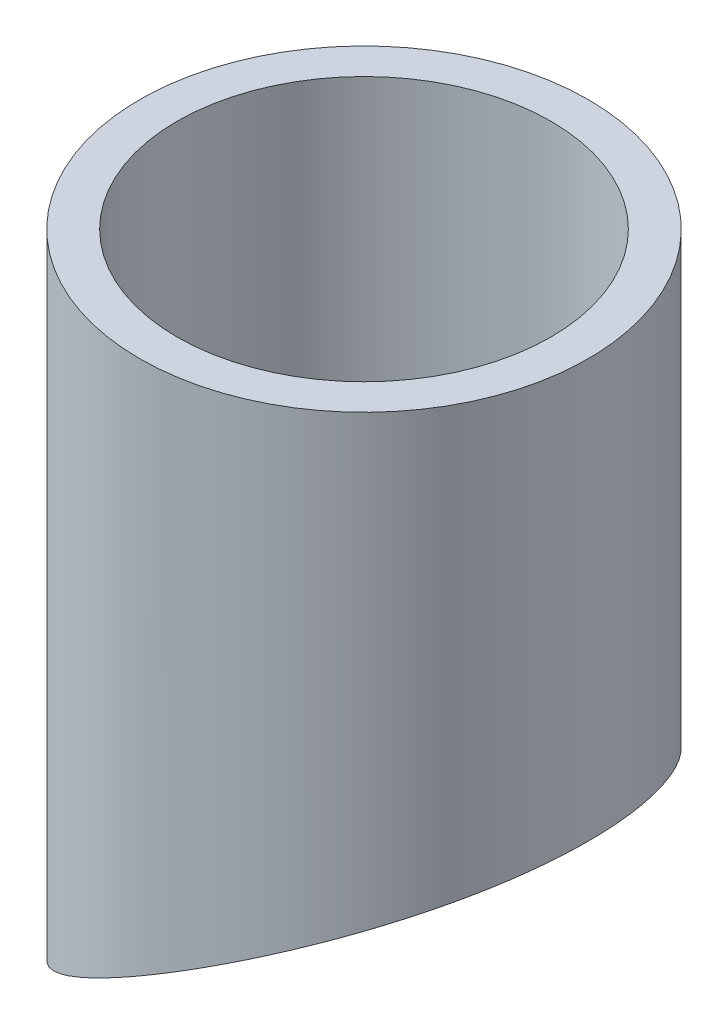
from build123d import *

# Parameters (mm, degrees)
SKETCH2_R               = 30
SKETCH2_R_2             = 25
BOSS_EXTRUDE1_DEPTH     = 400
CUT_EXTRUDE1_DEPTH      = 403.243707222
CUT_EXTRUDE1_DEPTH_BACK = 403.243707222
SKETCH3_R               = 379.5


with BuildPart() as part:
    # Sketch2 → Boss-Extrude1 (new body)
    with BuildSketch(Plane(origin=(0, 0, 0), x_dir=(1, 0, 0), z_dir=(0, 1, 0))):
        with Locations(Location((0, 0, 0), (0, 0, 270))):
            Circle(SKETCH2_R)
        with Locations(Location((0, 0, 0), (0, 0, 270))):
            Circle(SKETCH2_R_2, mode=Mode.SUBTRACT)
    extrude(amount=BOSS_EXTRUDE1_DEPTH)

    # Sketch3 → Cut-Extrude1 (cut, two sides: drawn at the far end of the back side and taken through both)
    with BuildSketch(Plane.XY.offset(-CUT_EXTRUDE1_DEPTH_BACK)):
        with Locations((190, 0)):
            Circle(SKETCH3_R)
    extrude(amount=CUT_EXTRUDE1_DEPTH + CUT_EXTRUDE1_DEPTH_BACK, mode=Mode.SUBTRACT)


solid = part.part
